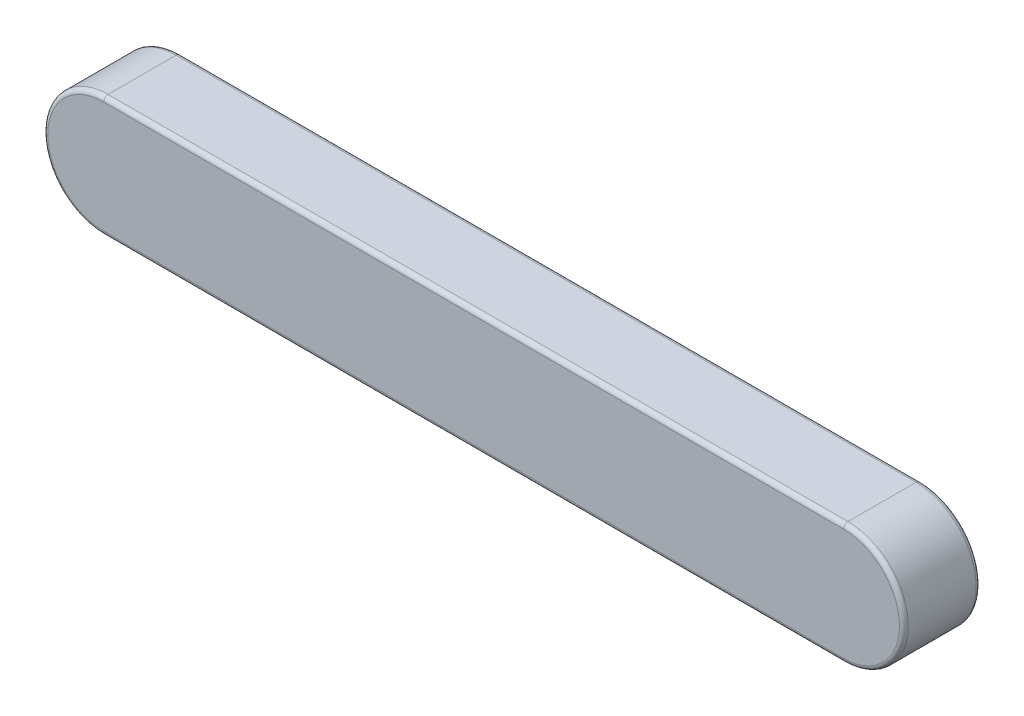
SolidWorks part; units mm, degrees
material "45"
ref_plane "Plane1" through (0, 0, 0) normal (0, 0, 1) x (1, 0, 0)
ref_plane "Plane2" through (0, 0, 0) normal (0, 1, 0) x (1, 0, 0)
ref_plane "Plane3" through (0, 0, 0) normal (1, 0, 0) x (0, 0, -1)
sketch "Sketch1" plane through (0, 0, 0) normal (0, 0, 1) x (1, 0, 0)
  line L0 (-14.6943, 0) -> (13.8107, 0) construction
  line L1 (-67.5, 11) -> (67.5, 11)
  line L2 (-67.5, -11) -> (67.5, -11)
  line L3 (0, 2.9108) -> (0, -2.1805) construction
  arc A0 (-67.5, 11) -> (-67.5, -11) centre (-67.5, 0) ccw
  arc A1 (67.5, 11) -> (67.5, -11) centre (67.5, 0) cw
  dimension "长度" = 157
  dimension "b" = 22
extrude "Boss-Extrude1" add sketch "Sketch1" along normal blind 14
fillet "Fillet1" radius 0.8 8 edges at (78.5, 0, 14) (0, 11, 14) (-78.5, 0, 14) (0, 11, 0) (78.5, 0, 0) (0, -11, 0) (-78.5, 0, 0) (0, -11, 14)
